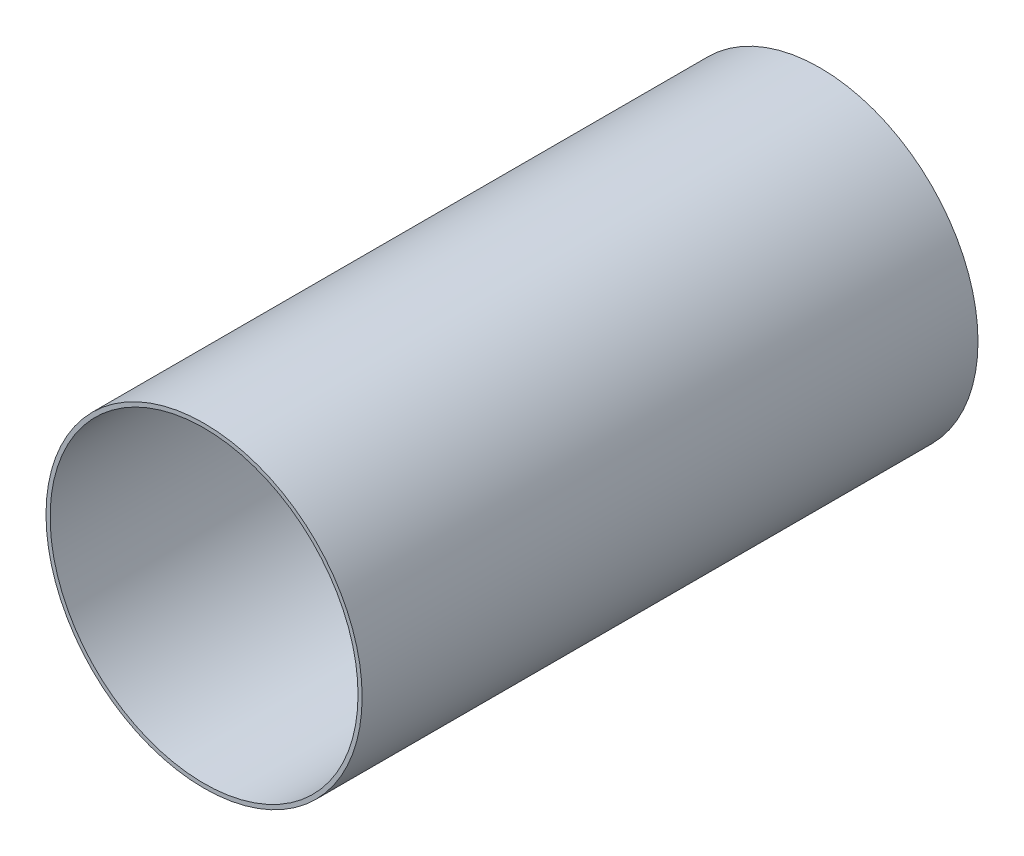
SolidWorks part; units mm, degrees
material "AISI 304"
ref_plane "Front Plane" through (0, 0, 0) normal (0, 0, 1) x (1, 0, 0)
ref_plane "Top Plane" through (0, 0, 0) normal (0, 1, 0) x (1, 0, 0)
ref_plane "Right Plane" through (0, 0, 0) normal (1, 0, 0) x (0, 0, -1)
sketch "Sketch1" plane through (0, 0, 0) normal (0, 0, 1) x (1, 0, 0)
  circle A0 centre (0, 0) radius 75
  circle A1 centre (0, 0) radius 77
  dimension "D1" = 150
  dimension "D2" = 154
extrude "Boss-Extrude1" add sketch "Sketch1" along normal blind 300
